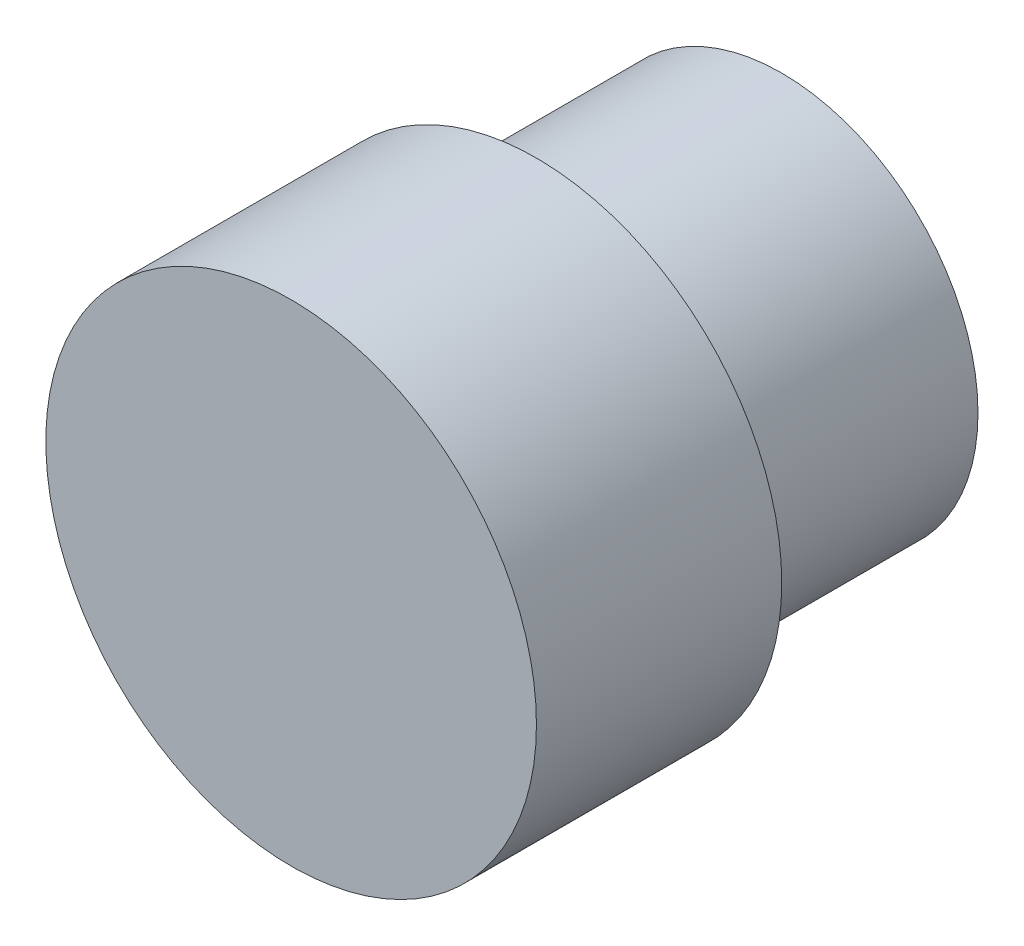
SolidWorks part; units mm, degrees
ref_plane "前视基准面" through (0, 0, 0) normal (0, 0, 1) x (1, 0, 0)
ref_plane "上视基准面" through (0, 0, 0) normal (0, 1, 0) x (1, 0, 0)
ref_plane "右视基准面" through (0, 0, 0) normal (1, 0, 0) x (0, 0, -1)
other "Configuration Table"
sketch "草图1" plane through (0, 0, 0) normal (0, 0, 1) x (1, 0, 0)
  circle A0 centre (0, 0) radius 8
  point P0 (0, 0)
  dimension "D1" = 16
extrude "凸台-拉伸1" add sketch "草图1" against normal blind 10
sketch "草图2" plane through (0, 0, 0) normal (0, 0, 1) x (1, 0, 0)
  circle A0 centre (0, 0) radius 10
  point P0 (0, 0)
  dimension "D1" = 20
extrude "凸台-拉伸2" add sketch "草图2" along normal blind 10
